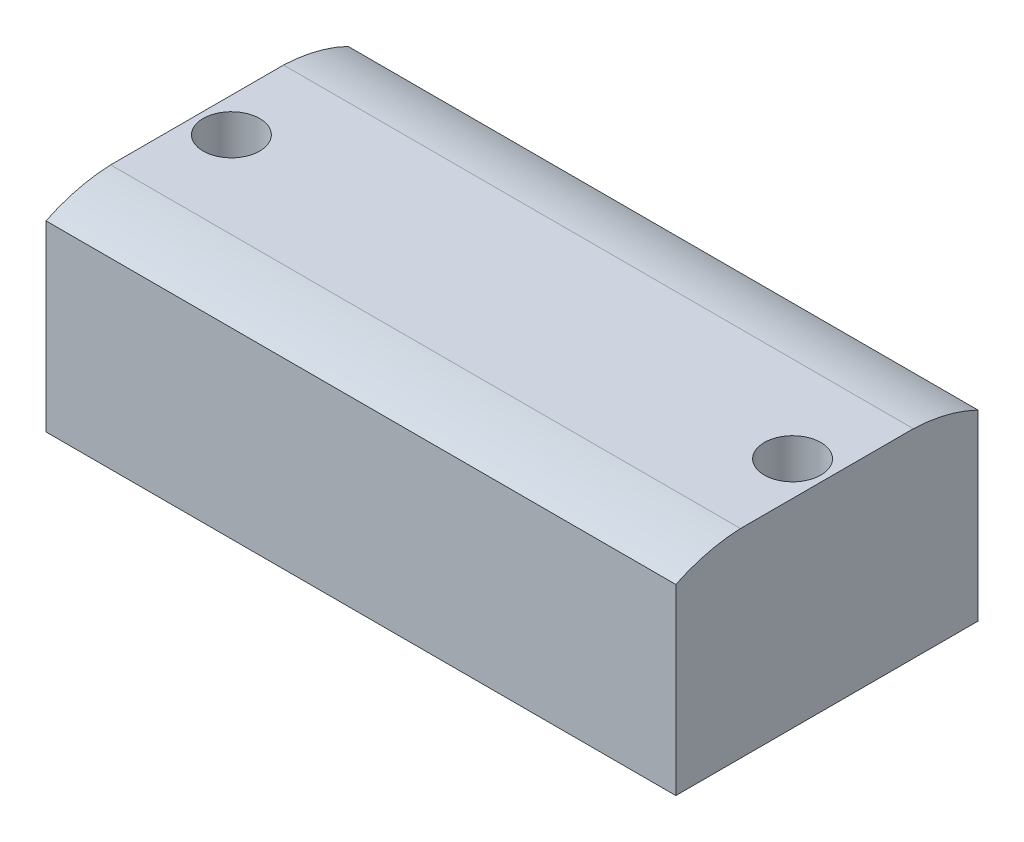
from build123d import *

# Parameters (mm, degrees)
SKETCH_1_W          = 77.96
SKETCH_1_H          = 24.63
EXTRUDE_1_DEPTH     = 18.7
CUT_EXTRUDE_1_DEPTH = 82.111718173
SKETCH_3_R          = 2.05
CUT_EXTRUDE_2_DEPTH = 50.757082913
SKETCH_4_R          = 3.5
CUT_EXTRUDE_3_DEPTH = 5


with BuildPart() as part:
    # 草图1 → 凸台-拉伸1 (new, symmetric)
    with BuildSketch(Plane.XY):
        Rectangle(SKETCH_1_W, SKETCH_1_H)
    extrude(amount=EXTRUDE_1_DEPTH, both=True)

    # 草图2 → 切除-拉伸1 (cut, through all)
    with BuildSketch(Plane(origin=(38.98, 0, 0), x_dir=(0, 0, -1), z_dir=(1, 0, 0))):
        with BuildLine():
            Line((-18.7, 10.315), (-18.7, 12.315))
            Line((-18.7, 12.315), (-10.7, 12.315))
            ThreePointArc((-10.7, 12.315), (-14.804196751, 11.731787003), (-18.7, 10.315))
        make_face()
        with BuildLine():
            Line((18.7, 12.315), (10.7, 12.315))
            ThreePointArc((10.7, 12.315), (14.804196751, 11.731787003), (18.7, 10.315))
            Line((18.7, 10.315), (18.7, 12.315))
        make_face()
    extrude(amount=-CUT_EXTRUDE_1_DEPTH, mode=Mode.SUBTRACT)

    # 草图3 → 切除-拉伸2 (cut, through all)
    with BuildSketch(Plane(origin=(0, 12.315, 0), x_dir=(1, 0, 0), z_dir=(0, 1, 0))):
        with Locations(Location((-34.73, 0, 0), (0, 0, 180))):
            Circle(SKETCH_3_R)
        with Locations((34.73, 0)):
            Circle(SKETCH_3_R)
    extrude(amount=-CUT_EXTRUDE_2_DEPTH, mode=Mode.SUBTRACT)

    # 草图4 → 切除-拉伸3 (cut)
    with BuildSketch(Plane(origin=(0, 12.315, 0), x_dir=(1, 0, 0), z_dir=(0, 1, 0))):
        with Locations(Location((-34.73, 0, 0), (0, 0, 180))):
            Circle(SKETCH_4_R)
        with Locations(Location((34.73, 0, 0), (0, 0, 180))):
            Circle(SKETCH_4_R)
    extrude(amount=-CUT_EXTRUDE_3_DEPTH, mode=Mode.SUBTRACT)


solid = part.part
